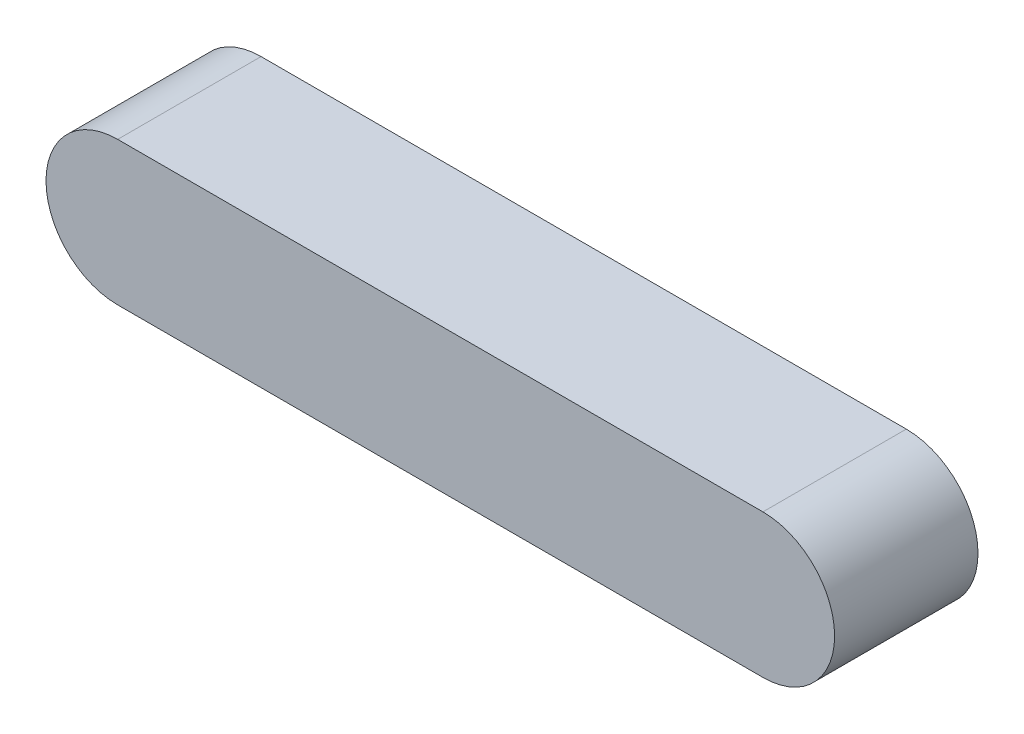
from build123d import *

# Parameters (mm, degrees)
BOSS_EXTRUDE1_DEPTH = 4


with BuildPart() as part:
    # Sketch1 → Boss-Extrude1 (new body)
    with BuildSketch(Plane.XY):
        with BuildLine():
            Line((0, 2), (18, 2))
            ThreePointArc((18, 2), (20, 0), (18, -2))
            Line((18, -2), (0, -2))
            ThreePointArc((0, -2), (-2, 0), (0, 2))
        make_face()
    extrude(amount=BOSS_EXTRUDE1_DEPTH)


solid = part.part
